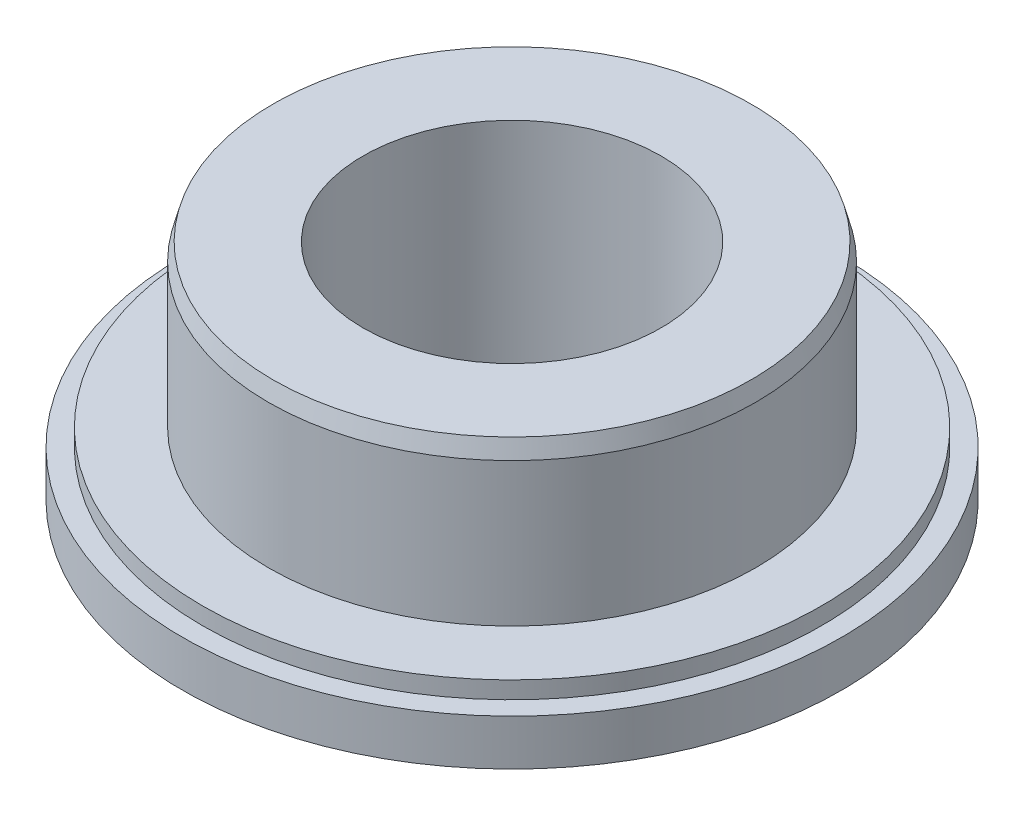
SolidWorks part; units mm, degrees
material "Q235"
ref_plane "Front Plane" through (0, 0, 0) normal (0, 0, 1) x (1, 0, 0)
ref_plane "Top Plane" through (0, 0, 0) normal (0, 1, 0) x (1, 0, 0)
ref_plane "Right Plane" through (0, 0, 0) normal (1, 0, 0) x (0, 0, -1)
sketch "Sketch1" plane through (0, 0, 0) normal (0, 0, 1) x (1, 0, 0)
  line L0 (26, 31) -> (42.5, 31)
  line L1 (42.5, 31) -> (42.5, 3)
  line L2 (42.5, 3) -> (54, 3)
  line L3 (54, 3) -> (54, 0)
  line L4 (54, 0) -> (57.5, 0)
  line L5 (57.5, 0) -> (57.5, -8)
  line L6 (57.5, -8) -> (26, -8)
  line L7 (26, -8) -> (26, 31)
  line L8 (0, 0) -> (0, 41.1083) construction
  dimension "D1" = 42.5
  dimension "D2" = 54
  dimension "D3" = 57.5
  dimension "D4" = 28
  dimension "D5" = 3
  dimension "D6" = 8
  dimension "D7" = 26
revolve "Revolve1" add sketch "Sketch1" angle 360 about L8
chamfer "Chamfer1" distance 3 angle 15 1 edges at (0, 31, -42.5)
